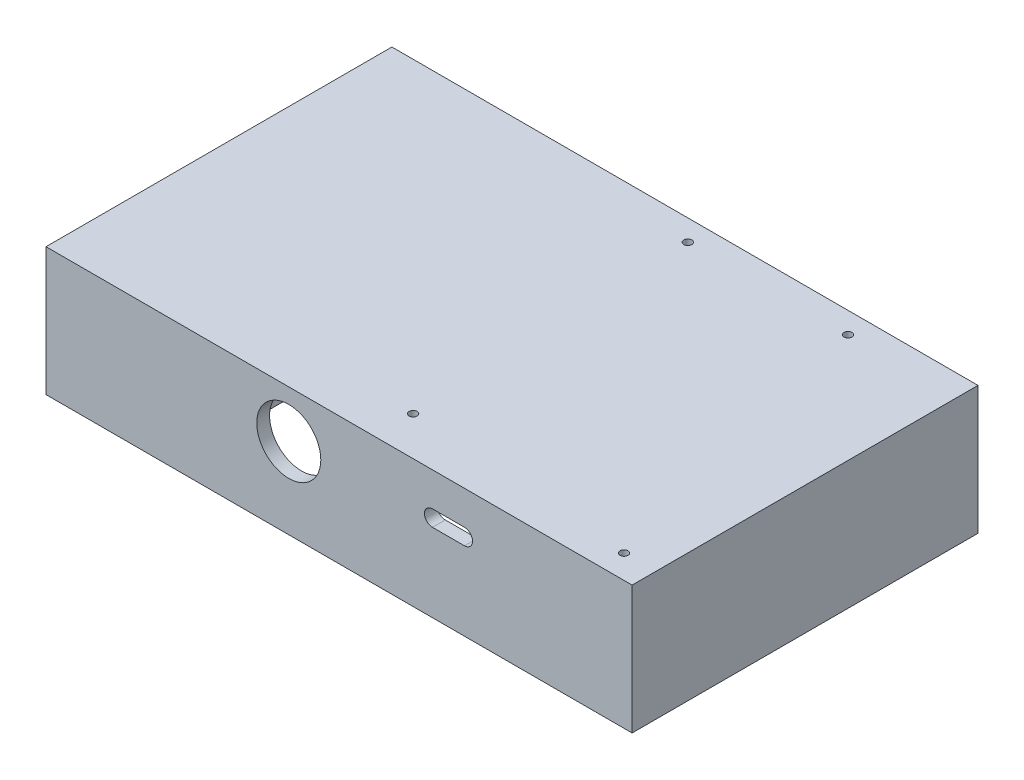
from build123d import *

# Parameters (mm, degrees)
SKETCH2_W               = 366
SKETCH2_H               = 216
SKETCH2_W_2             = 350
SKETCH2_H_2             = 200
BOSS_EXTRUDE1_DEPTH     = 80
SKETCH4_W               = 350
SKETCH4_H               = 200
BOSS_EXTRUDE2_DEPTH     = 2
CUT_EXTRUDE1_DEPTH      = 61
SKETCH6_W               = 120
SKETCH6_H               = 50
CUT_EXTRUDE2_DEPTH      = 61
SKETCH7_R               = 5
SKETCH7_R_2             = 2.5
BOSS_EXTRUDE6_DEPTH     = 11
SKETCH8_R               = 2.5
CUT_EXTRUDE3_DEPTH      = 223.804847344
SKETCH10_R              = 5
BOSS_EXTRUDE7_DEPTH     = 11
SKETCH9_R               = 5
BOSS_EXTRUDE8_DEPTH     = 11
SKETCH11_R              = 2.5
CUT_EXTRUDE4_DEPTH      = 223.804847344
SKETCH12_W              = 2
SKETCH12_H              = 200
EXTRUDE_THIN1_DEPTH     = 66
SKETCH14_W              = 79.91
SKETCH14_H              = 45
BOSS_EXTRUDE9_DEPTH     = 2
LPATTERN1_COUNT         = 3
LPATTERN1_PITCH         = 50
CUT_EXTRUDE5_DEPTH      = 114
CUT_EXTRUDE5_DEPTH_BACK = 26
SKETCH15_R              = 33.472147388
SKETCH16_R              = 20
CUT_EXTRUDE6_DEPTH      = 114
SKETCH20_W              = 113.827039933
SKETCH20_H              = 27.666294428
BOSS_EXTRUDE12_DEPTH    = 41
SKETCH21_R              = 4.720605869
BOSS_EXTRUDE13_DEPTH    = 10


with BuildPart() as part:
    # Sketch2 → Boss-Extrude1 (new body)
    with BuildSketch(Plane(origin=(0, 0, 0), x_dir=(1, 0, 0), z_dir=(0, 1, 0))):
        Rectangle(SKETCH2_W, SKETCH2_H)
        Rectangle(SKETCH2_W_2, SKETCH2_H_2, mode=Mode.SUBTRACT)
    extrude(amount=BOSS_EXTRUDE1_DEPTH)

    # Sketch4 → Boss-Extrude2 (add)
    with BuildSketch(Plane(origin=(0, 80, 0), x_dir=(1, 0, 0), z_dir=(0, 1, 0))):
        Rectangle(SKETCH4_W, SKETCH4_H)
    extrude(amount=-BOSS_EXTRUDE2_DEPTH)

    # Sketch5 → Cut-Extrude1 (cut, symmetric)
    with BuildSketch(Plane.XY.offset(108)):
        with BuildLine():
            Line((58.33950225, 58.901074255), (78.33950225, 58.901074255))
            ThreePointArc((78.33950225, 58.901074255), (83.33950225, 53.901074255), (78.33950225, 48.901074255))
            Line((78.33950225, 48.901074255), (58.33950225, 48.901074255))
            ThreePointArc((58.33950225, 48.901074255), (53.33950225, 53.901074255), (58.33950225, 58.901074255))
        make_face()
    extrude(amount=CUT_EXTRUDE1_DEPTH, both=True, mode=Mode.SUBTRACT)

    # Sketch6 → Cut-Extrude2 (cut, symmetric)
    with BuildSketch(Plane.XY.offset(-100)):
        with Locations((-0.151988162, 42.065744544)):
            Rectangle(SKETCH6_W, SKETCH6_H)
    extrude(amount=CUT_EXTRUDE2_DEPTH, both=True, mode=Mode.SUBTRACT)

    # Sketch7 → Boss-Extrude6 (add)
    # profile 1 of 2: a face of its own
    with BuildSketch(Plane.XZ.offset(-78)):
        with Locations(Location((115, -94.8, 0), (0, 0, 90))):
            Circle(SKETCH7_R)
        with Locations(Location((115, -94.8, 0), (0, 0, 270))):
            Circle(SKETCH7_R_2, mode=Mode.SUBTRACT)
    # profile 2 of 2: a face of its own
    with BuildSketch(Plane.XZ.offset(-78)):
        with Locations(Location((15, -94.8, 0), (0, 0, 90))):
            Circle(SKETCH7_R)
        with Locations(Location((15, -94.8, 0), (0, 0, 270))):
            Circle(SKETCH7_R_2, mode=Mode.SUBTRACT)
    extrude(amount=BOSS_EXTRUDE6_DEPTH)

    # Sketch8 → Cut-Extrude3 (cut, through all)
    with BuildSketch(Plane.XZ.offset(-67)):
        with Locations(Location((15, -94.8, 0), (0, 0, 270))):
            Circle(SKETCH8_R)
        with Locations(Location((115, -94.8, 0), (0, 0, 270))):
            Circle(SKETCH8_R)
    extrude(amount=-CUT_EXTRUDE3_DEPTH, mode=Mode.SUBTRACT)

    # Sketch10 → Boss-Extrude7 (add)
    with BuildSketch(Plane.XZ.offset(-78)):
        with Locations(Location((163.162408198, 93.199516901, 0), (0, 0, 90))):
            Circle(SKETCH10_R)
    extrude(amount=BOSS_EXTRUDE7_DEPTH)

    # Sketch9 → Boss-Extrude8 (add)
    with BuildSketch(Plane.XZ.offset(-78)):
        with Locations(Location((21.965532886, 83.705206519, 0), (0, 0, 90))):
            Circle(SKETCH9_R)
    extrude(amount=BOSS_EXTRUDE8_DEPTH)

    # Sketch11 → Cut-Extrude4 (cut, through all)
    with BuildSketch(Plane.XZ.offset(-67)):
        with Locations(Location((21.965532886, 83.705206519, 0), (0, 0, 270))):
            Circle(SKETCH11_R)
        with Locations(Location((163.162408198, 93.199516901, 0), (0, 0, 270))):
            Circle(SKETCH11_R)
    extrude(amount=-CUT_EXTRUDE4_DEPTH, mode=Mode.SUBTRACT)

    # Sketch12 → Extrude-Thin1 (add)
    with BuildSketch(Plane.XZ.offset(-78)):
        with Locations((-94.091079546, 0)):
            Rectangle(SKETCH12_W, SKETCH12_H)
    extrude(amount=EXTRUDE_THIN1_DEPTH)

    # Sketch14 → Boss-Extrude9 (add, symmetric)
    with BuildSketch(Plane.XY.offset(40)):
        with Locations((-134.390971406, 55.5)):
            Rectangle(SKETCH14_W, SKETCH14_H)
    boss_extrude9 = extrude(amount=BOSS_EXTRUDE9_DEPTH, both=True)

    # LPattern1: Boss-Extrude9 ×3
    with Locations(*[(0, 0, -i * LPATTERN1_PITCH) for i in range(1, LPATTERN1_COUNT)]):
        add(boss_extrude9)

    # Sketch15 → Cut-Extrude5 (cut, two sides: drawn at the far end of the back side and taken through both)
    with BuildSketch(Plane(origin=(0, 0, 38), x_dir=(-1, 0, 0), z_dir=(0, 0, -1)).offset(-CUT_EXTRUDE5_DEPTH_BACK)):
        with Locations((134.390971406, 39.071496759)):
            Circle(SKETCH15_R)
    extrude(amount=CUT_EXTRUDE5_DEPTH + CUT_EXTRUDE5_DEPTH_BACK, mode=Mode.SUBTRACT)

    # Sketch16 → Cut-Extrude6 (cut)
    with BuildSketch(Plane.XY.offset(108)):
        with Locations((-31.393490916, 50.490695355)):
            Circle(SKETCH16_R)
    extrude(amount=-CUT_EXTRUDE6_DEPTH, mode=Mode.SUBTRACT)

    # Sketch20 → Boss-Extrude12 (add)
    with BuildSketch(Plane.XZ.offset(-78)):
        with Locations((7.170460987, -56.94888764)):
            Rectangle(SKETCH20_W, SKETCH20_H)
    extrude(amount=BOSS_EXTRUDE12_DEPTH)

    # Sketch21 → Boss-Extrude13 (add)
    with BuildSketch(Plane(origin=(0, 0, -70.782034854), x_dir=(-1, 0, 0), z_dir=(0, 0, -1))):
        with Locations(Location((-47.399149027, 53.301801825, 0), (0, 0, 180))):
            Circle(SKETCH21_R)
        with Locations(Location((-23.290302455, 53.301801825, 0), (0, 0, 180))):
            Circle(SKETCH21_R)
        with Locations(Location((5.245340735, 53.301801825, 0), (0, 0, 180))):
            Circle(SKETCH21_R)
        with Locations(Location((26.829705026, 53.301801825, 0), (0, 0, 180))):
            Circle(SKETCH21_R)
    extrude(amount=BOSS_EXTRUDE13_DEPTH)


solid = part.part
